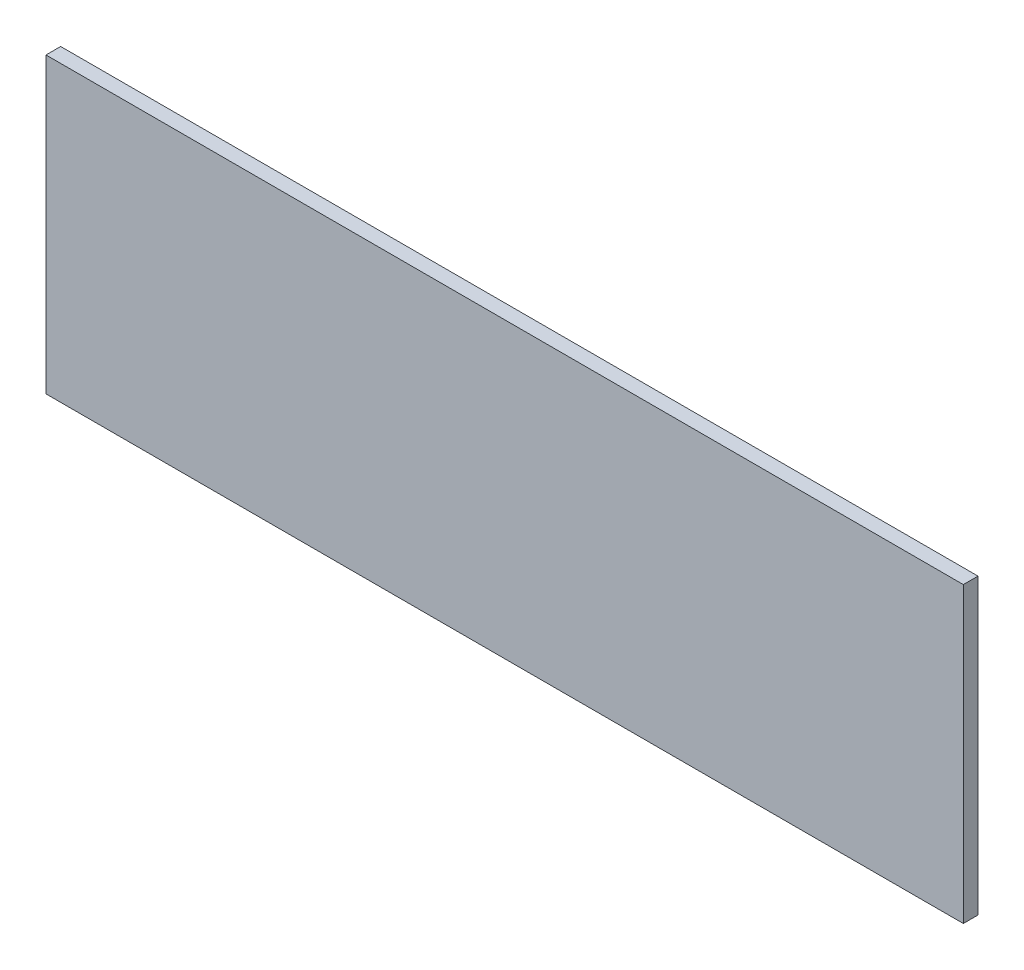
SolidWorks part; units mm, degrees
material "Q235-A"
ref_plane "前视基准面" through (0, 0, 0) normal (0, 0, 1) x (1, 0, 0)
ref_plane "上视基准面" through (0, 0, 0) normal (0, 1, 0) x (1, 0, 0)
ref_plane "右视基准面" through (0, 0, 0) normal (1, 0, 0) x (0, 0, -1)
sketch "草图1" plane through (0, 0, 0) normal (0, 0, 1) x (1, 0, 0)
  line L0 (0, 20) -> (0, -20) construction
  line L1 (-62.5, 20) -> (62.5, 20)
  line L2 (-62.5, 20) -> (-62.5, -20)
  line L3 (-62.5, -20) -> (62.5, -20)
  line L4 (62.5, 20) -> (62.5, -20)
  point P6 (0, 0)
  dimension "D1" = 40
  dimension "D2" = 125
extrude "凸台-拉伸1" add sketch "草图1" along normal blind 2
